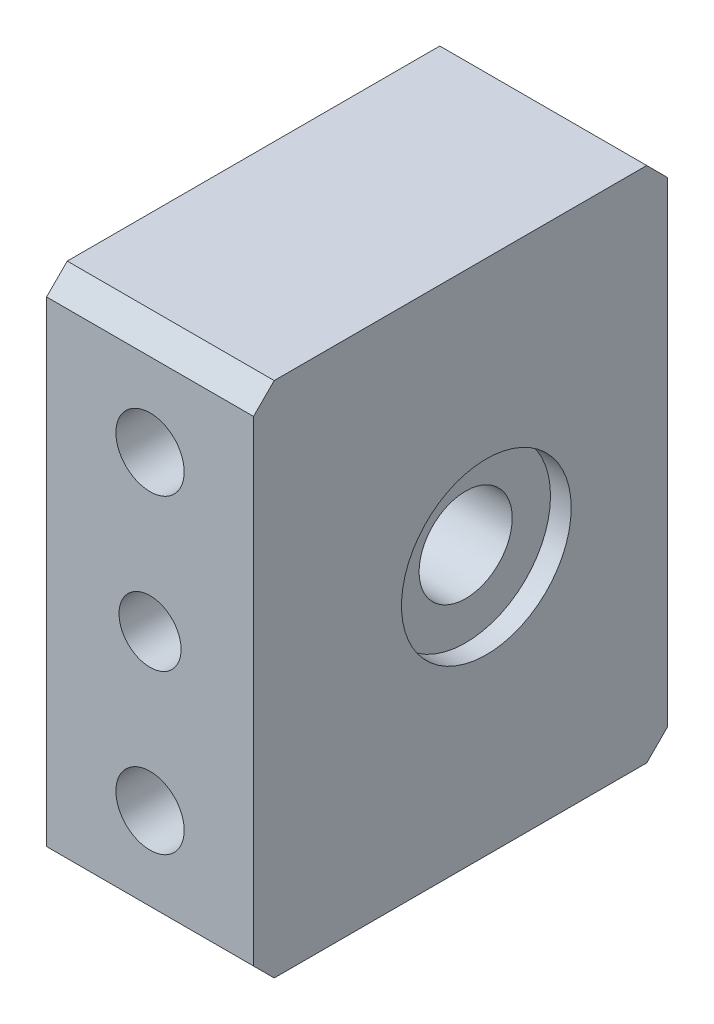
from build123d import *

# Parameters (mm, degrees)
SKETCH_1_W                = 10
SKETCH_1_H                = 20
EXTRUDE_1_DEPTH           = 25
HOLE_WIZARD_1_D           = 4.5
HOLE_WIZARD_1_DEPTH       = 10.1
HOLE_WIZARD_1_CBORE_D     = 8
HOLE_WIZARD_1_CBORE_DEPTH = 4.6
HOLE_WIZARD_1_TIP         = 1.351936393
SKETCH_4_R                = 4.1
CUT_EXTRUDE_1_DEPTH       = 1
HOLE_WIZARD_M4_1_D        = 3.3
HOLE_WIZARD_M4_1_DEPTH    = 10.1
HOLE_WIZARD_M4_1_TIP      = 0.991420021
MM_1_D                    = 3
MM_1_DEPTH                = 6
MM_1_TIP                  = 0.901290929
CHAMFER_1_SIZE            = 1


with BuildPart() as part:
    # 草图1 → 凸台-拉伸1 (new body)
    with BuildSketch(Plane(origin=(0, 0, 0), x_dir=(1, 0, 0), z_dir=(0, 1, 0))):
        Rectangle(SKETCH_1_W, SKETCH_1_H)
    extrude(amount=EXTRUDE_1_DEPTH)

    # 打孔尺寸(%根据)内六角圆柱头螺钉的类型1
    with Locations(Plane.ZY.offset(5)):
        with Locations((-1.25, 12.5)):
            CounterBoreHole(HOLE_WIZARD_1_D / 2, HOLE_WIZARD_1_CBORE_D / 2, HOLE_WIZARD_1_CBORE_DEPTH, depth=HOLE_WIZARD_1_DEPTH)
            with Locations((0, 0, -(HOLE_WIZARD_1_DEPTH + HOLE_WIZARD_1_TIP / 2))):  # 118° drill point
                Cone(0, HOLE_WIZARD_1_D / 2, HOLE_WIZARD_1_TIP, mode=Mode.SUBTRACT)

    # 草图4 → 切除-拉伸1 (cut)
    with BuildSketch(Plane(origin=(5, 0, 0), x_dir=(0, 0, -1), z_dir=(1, 0, 0))):
        with Locations((1.25, 12.5)):
            Circle(SKETCH_4_R)
    extrude(amount=-CUT_EXTRUDE_1_DEPTH, mode=Mode.SUBTRACT)

    # M4 螺纹孔1
    with Locations(Plane.XY.offset(10)):
        with Locations((0, 20), (0, 5)):
            Hole(HOLE_WIZARD_M4_1_D / 2, depth=HOLE_WIZARD_M4_1_DEPTH)
            with Locations((0, 0, -(HOLE_WIZARD_M4_1_DEPTH + HOLE_WIZARD_M4_1_TIP / 2))):  # 118° drill point
                Cone(0, HOLE_WIZARD_M4_1_D / 2, HOLE_WIZARD_M4_1_TIP, mode=Mode.SUBTRACT)

    # 大小mm 暗销孔1
    with Locations(Plane.XY.offset(10)):
        with Locations((0, 12.5)):
            Hole(MM_1_D / 2, depth=MM_1_DEPTH)
            with Locations((0, 0, -(MM_1_DEPTH + MM_1_TIP / 2))):  # 118° drill point
                Cone(0, MM_1_D / 2, MM_1_TIP, mode=Mode.SUBTRACT)

    # 倒角1
    chamfer_1_edges = [part.edges().sort_by_distance(p)[0] for p in [
        (0, 25, 10),
        (0, 0, 10),
        (0, 0, -10),
        (0, 25, -10),
    ]]
    chamfer(chamfer_1_edges, length=CHAMFER_1_SIZE)


solid = part.part
